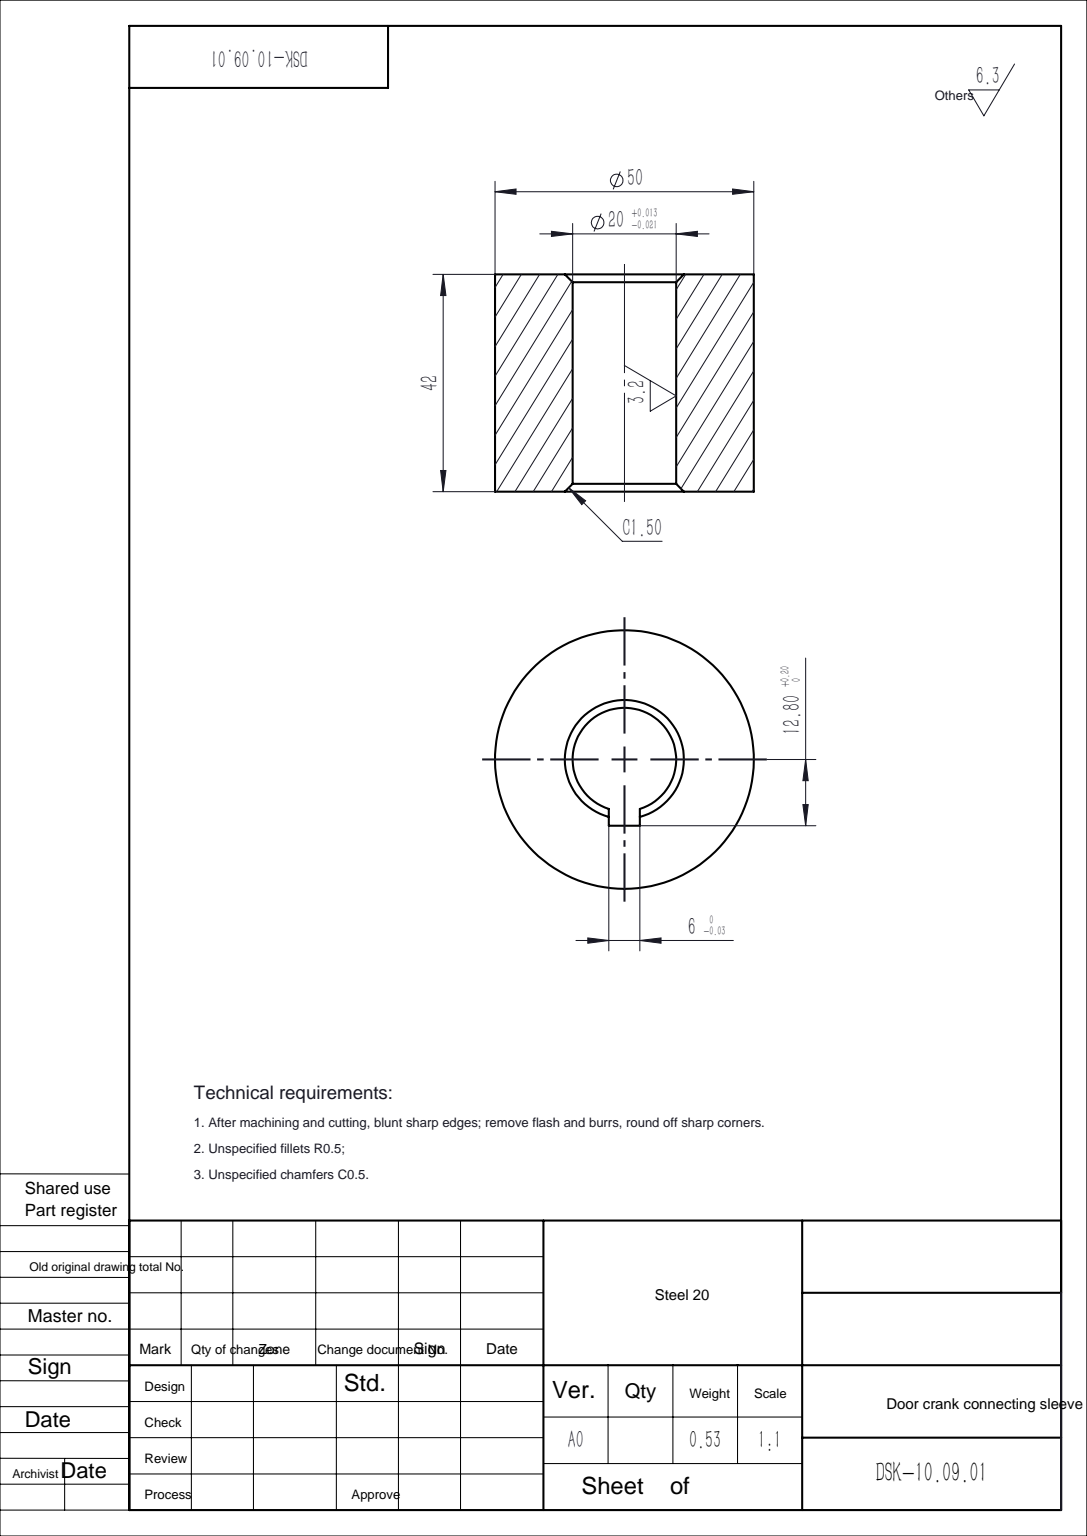
from build123d import *

# Parameters (mm, degrees)
SKETCH1_R           = 25
BOSS_EXTRUDE1_DEPTH = 42
CHAMFER1_SIZE       = 1.5


with BuildPart() as part:
    # Sketch1 → Boss-Extrude1 (new body)
    with BuildSketch(Plane(origin=(0, 0, 0), x_dir=(1, 0, 0), z_dir=(0, 1, 0))):
        with Locations(Location((0, 0, 0), (0, 0, 90))):
            Circle(SKETCH1_R)
        with BuildLine():
            ThreePointArc((10, 0), (8.062257748, -5.916079783), (3, -9.539392014))
            Line((3, -9.539392014), (3, -12.8))
            Line((3, -12.8), (-3, -12.8))
            Line((-3, -12.8), (-3, -9.539392014))
            ThreePointArc((-3, -9.539392014), (-5.916079783, 8.062257748), (10, 0))
        make_face(mode=Mode.SUBTRACT)
    extrude(amount=BOSS_EXTRUDE1_DEPTH)

    # Chamfer1
    chamfer1_edges = [part.edges().sort_by_distance(p)[0] for p in [
        (-5.916079783, 42, -8.062257748),
        (-5.916079783, 0, -8.062257748),
    ]]
    chamfer(chamfer1_edges, length=CHAMFER1_SIZE)


solid = part.part
